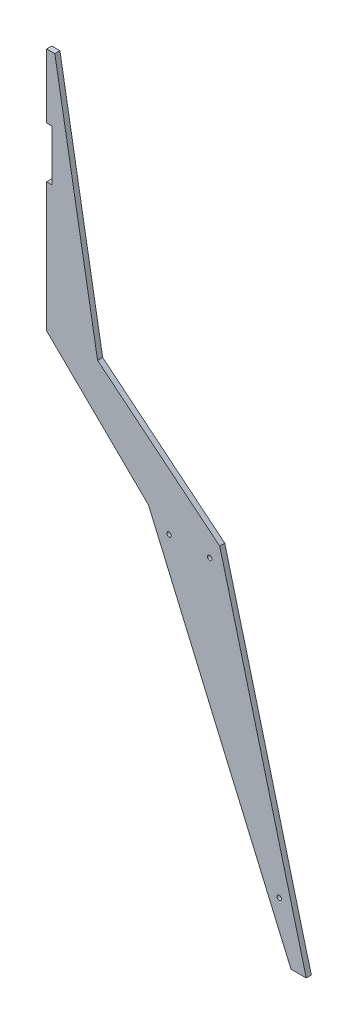
SolidWorks part; units mm, degrees
ref_plane "前视基准面" through (0, 0, 0) normal (0, 0, 1) x (1, 0, 0)
ref_plane "上视基准面" through (0, 0, 0) normal (0, 1, 0) x (1, 0, 0)
ref_plane "右视基准面" through (0, 0, 0) normal (1, 0, 0) x (0, 0, -1)
sketch "草图1" plane through (0, 0, 0) normal (0, 0, 1) x (1, 0, 0)
  line L0 (0, 0) -> (8, 0)
  line L1 (8, 0) -> (50, -240)
  line L2 (50, -240) -> (170, -338)
  line L3 (170, -338) -> (255, -663)
  line L4 (255, -663) -> (240, -663)
  line L5 (240, -663) -> (100, -338)
  line L6 (100, -338) -> (0, -240)
  line L8 (0, -240) -> (0, -113)
  line L9 (0, -113) -> (5, -113)
  line L10 (5, -113) -> (5, -63)
  line L11 (5, -63) -> (0, -63)
  line L12 (0, -63) -> (0, 0)
  line L13 (100, -338) -> (170, -338) construction
  line L14 (50, -240) -> (0, -240) construction
  dimension "D1" = 8
  dimension "D2" = 63
  dimension "D3" = 5
  dimension "D4" = 50
  dimension "D5" = 15
  dimension "D6" = 255
  dimension "D7" = 50
  dimension "D8" = 98
  dimension "D9" = 240
  dimension "D10" = 325
  dimension "D11" = 170
  dimension "D12" = 70
extrude "凸台-拉伸1" add sketch "草图1" along normal mid plane 5
sketch "草图2" plane through (0, 0, 2.5) normal (0, 0, 1) x (1, 0, 0)
  line L0 (100, -338) -> (170, -338) construction
  line L1 (135, -338) -> (247.5, -663) construction
  line L2 (120.1923, -353) -> (160.1923, -353) construction
  line L3 (240, -663) -> (255, -663) construction
  circle A0 centre (120.1923, -353) radius 2.2
  circle A1 centre (160.1923, -353) radius 2.2
  point P10 (140.1923, -353)
  dimension "D1" = 4.4
  dimension "D2" = 15
  dimension "D3" = 40
extrude "切除-拉伸1" cut sketch "草图2" against normal blind 10
sketch "草图3" plane through (0, 0, 2.5) normal (0, 0, 1) x (1, 0, 0)
  circle A0 centre (228.4615, -608) radius 2.2 construction
  circle A1 centre (228.4615, -608) radius 2.2
extrude "切除-拉伸2" cut sketch "草图3" against normal blind 10
